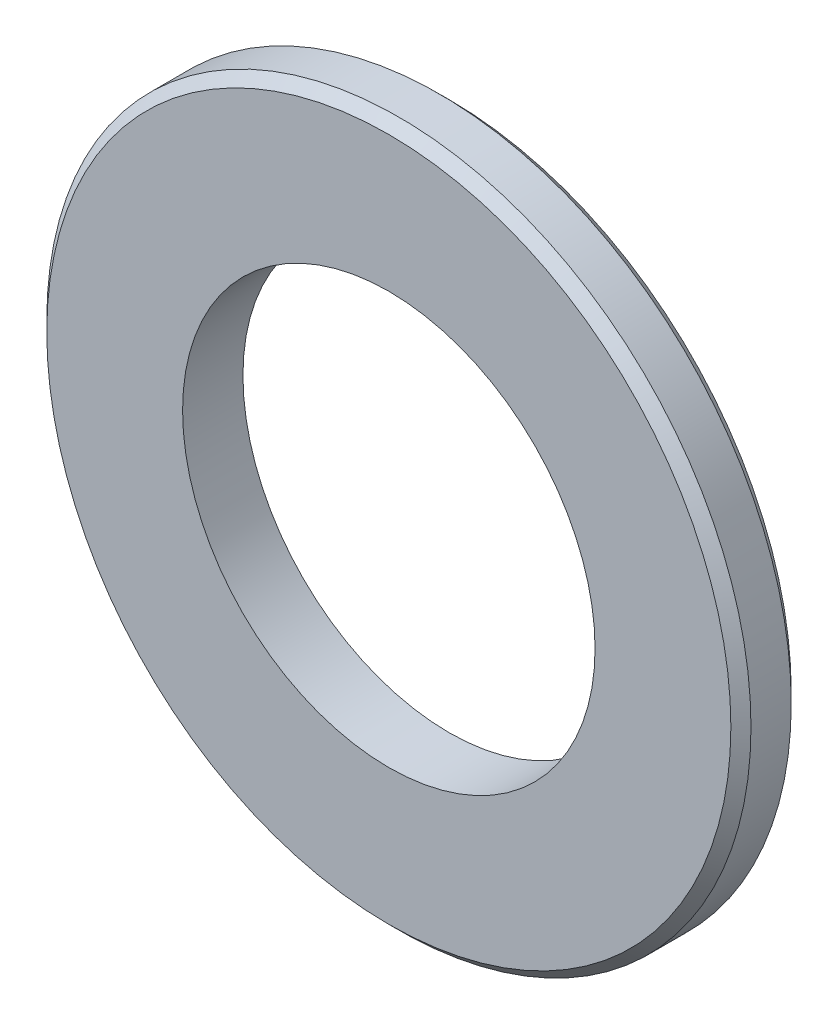
from build123d import *

# Parameters (mm, degrees)
SKETCH_1_R      = 17.5
SKETCH_1_R_2    = 10.25
EXTRUDE_1_DEPTH = 3
CHAMFER_1_SIZE  = 0.5


with BuildPart() as part:
    # 草图1 → 凸台-拉伸1 (new body)
    with BuildSketch(Plane.XY):
        Circle(SKETCH_1_R)
        Circle(SKETCH_1_R_2, mode=Mode.SUBTRACT)
    extrude(amount=EXTRUDE_1_DEPTH)

    # 倒角1
    chamfer_1_edges = [part.edges().sort_by_distance(p)[0] for p in [
        (-17.5, 0, 0),
        (-17.5, 0, 3),
    ]]
    chamfer(chamfer_1_edges, length=CHAMFER_1_SIZE)


solid = part.part
